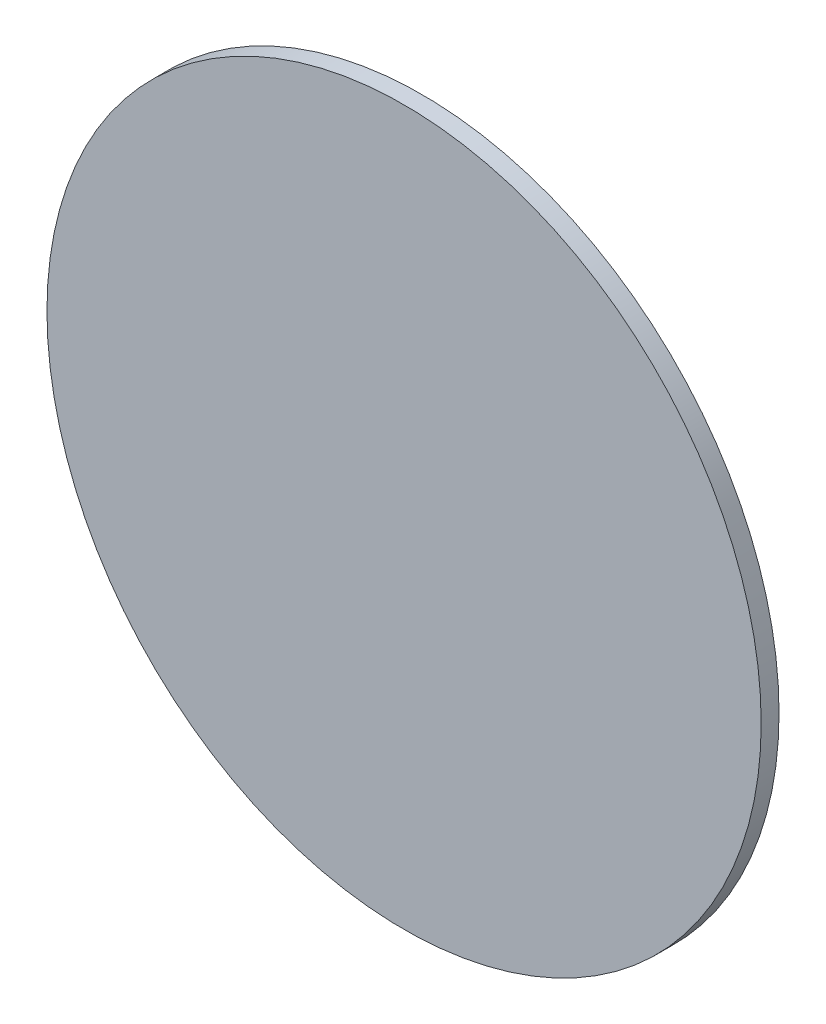
SolidWorks part; units mm, degrees
material "1023 碳钢板 (SS)"
ref_plane "Front Plane" through (0, 0, 0) normal (0, 0, 1) x (1, 0, 0)
ref_plane "Top Plane" through (0, 0, 0) normal (0, 1, 0) x (1, 0, 0)
ref_plane "Right Plane" through (0, 0, 0) normal (1, 0, 0) x (0, 0, -1)
sketch "Sketch1" plane through (0, 0, 0) normal (0, 0, 1) x (1, 0, 0)
  circle A0 centre (0, 0) radius 20
extrude "Boss-Extrude1" add sketch "Sketch1" along normal blind 1
sketch "Sketch2" plane through (0, 0, 0) normal (0, 0, -1) x (-1, 0, 0)
  circle A0 centre (0, 0) radius 2
extrude "Boss-Extrude2" add sketch "Sketch2" along normal blind 1
sketch "Sketch3" plane through (0, 0, -1) normal (0, 0, -1) x (-1, 0, 0)
  circle A0 centre (0, 0) radius 12.5
extrude "Boss-Extrude3" add sketch "Sketch3" along normal blind 1
